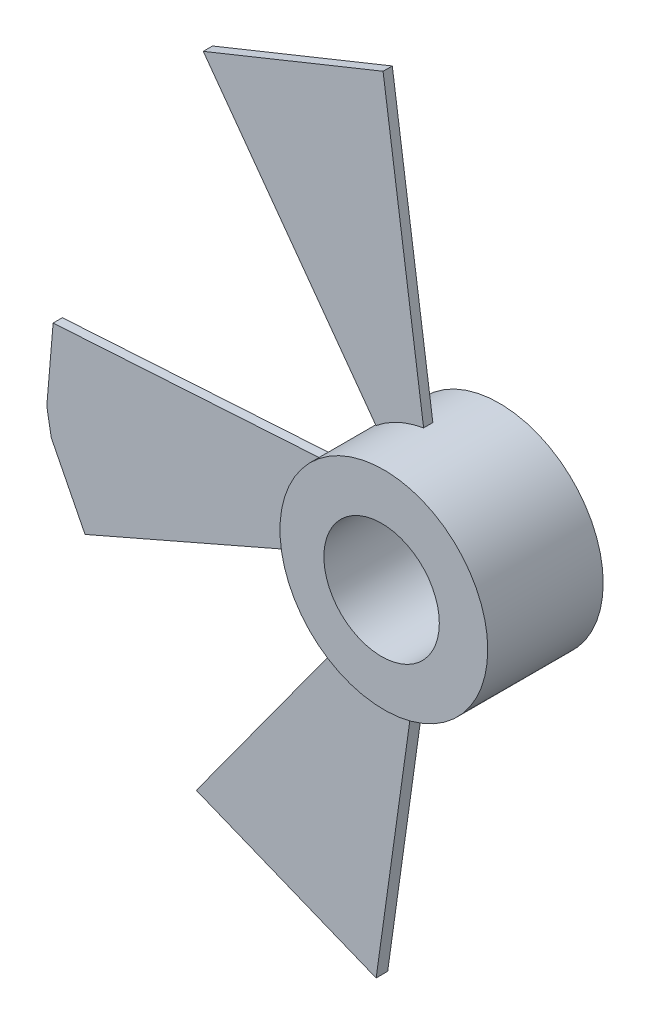
from build123d import *

# Parameters (mm, degrees)
EXTRUDE_1_DEPTH     = 4
EXTRUDE_1_2_DEPTH   = 4
EXTRUDE_1_3_DEPTH   = 4
SKETCH_2_R          = 90
SKETCH_2_R_2        = 57.5
EXTRUDE_2_DEPTH     = 50
SKETCH_4_R          = 57.5
SKETCH_4_R_2        = 50
EXTRUDE_3_DEPTH     = 100
CUT_EXTRUDE_1_DEPTH = 485.810454508
EXTRUDE_START       = 10
EXTRUDE_4_DEPTH     = 10


with BuildPart() as part:
    # 草图1 → 凸台-拉伸1 (new, symmetric)
    with BuildSketch(Plane.XY):
        with BuildLine():
            Line((-10.924807901, 55.668937127), (-50.690571005, 338.617043901))
            Line((-50.690571005, 338.617043901), (-206.438031879, 275.690985101))
            Line((-206.438031879, 275.690985101), (-37.918188894, 43.743319974))
            ThreePointArc((-37.918188894, 43.743319974), (-25.199590106, 51.467322598), (-10.924807901, 55.668937127))
        make_face()
    extrude(amount=EXTRUDE_1_DEPTH, both=True)



with BuildPart() as body_2:
    # 草图1 → Extrude 1 2 (new, symmetric)
    with BuildSketch(Plane.XY):
        with BuildLine():
            Line((-341.966631122, -58.160848878), (-338.146174396, -79.914727665))
            Line((-338.146174396, -79.914727665), (-308.839134252, -137.932805865))
            Line((-308.839134252, -137.932805865), (-53.490261468, -26.646674297))
            ThreePointArc((-53.490261468, -26.646674297), (-59.462925063, -1.128374922), (-53.490261468, 24.389924453))
            Line((-53.490261468, 24.389924453), (-336.508428621, 6.839151122))
            Line((-336.508428621, 6.839151122), (-341.966631122, -58.160848878))
        make_face()
    extrude(amount=EXTRUDE_1_2_DEPTH, both=True)


with BuildPart() as body_3:
    # 草图1 → Extrude 1 3 (new, symmetric)
    with BuildSketch(Plane.XY):
        with BuildLine():
            Line((-14.977351718, -57.136184189), (-46.962925063, -340))
            Line((-46.962925063, -340), (68.037074937, -340))
            Line((68.037074937, -340), (24.752563392, -52.045294277))
            ThreePointArc((24.752563392, -52.045294277), (5.345225431, -58.162057394), (-14.977351718, -57.136184189))
        make_face()
    extrude(amount=EXTRUDE_1_3_DEPTH, both=True)


with BuildPart() as part_1:
    add(part.part)

    add(body_2.part)  # 凸台-拉伸2 merges body 2

    add(body_3.part)  # 凸台-拉伸2 merges body 3
    # 草图2 → 凸台-拉伸2 (add, symmetric)
    with BuildSketch(Plane.XY.offset(4)):
        Circle(SKETCH_2_R)
        with Locations((-1.962925063, -1.128374922)):
            Circle(SKETCH_2_R_2, mode=Mode.SUBTRACT)
    extrude(amount=EXTRUDE_2_DEPTH, both=True)

    # 草图4 → 凸台-拉伸3 (add)
    with BuildSketch(Plane.XY.offset(54)):
        with Locations((-1.962925063, -1.128374922)):
            Circle(SKETCH_4_R)
        with Locations((-1.962925063, -1.128374922)):
            Circle(SKETCH_4_R_2, mode=Mode.SUBTRACT)
    extrude(amount=-EXTRUDE_3_DEPTH)

    # 草图7 → 切除-拉伸1 (cut, through all)
    with BuildSketch(Plane.XY.offset(4)):
        with BuildLine():
            Line((-18.476741558, -88.082972369), (-46.962925063, -340))
            Line((-46.962925063, -340), (68.037074937, -340))
            Line((68.037074937, -340), (29.699950595, -84.958301152))
            ThreePointArc((29.699950595, -84.958301152), (5.825032002, -89.811296629), (-18.476741558, -88.082972369))
        make_face()
    extrude(amount=-CUT_EXTRUDE_1_DEPTH, mode=Mode.SUBTRACT)

    # 草图9 → 凸台-拉伸4 (add)
    with BuildSketch(Plane.XY.offset(EXTRUDE_START)):
        with BuildLine():
            Line((-206.438031879, -275.690985101), (-56.836712635, -69.782434014))
            ThreePointArc((-56.836712635, -69.782434014), (-37.406446529, -81.858156332), (-15.559269973, -88.644848231))
            Line((-15.559269973, -88.644848231), (-50.690571005, -338.617043901))
            Line((-50.690571005, -338.617043901), (-206.438031879, -275.690985101))
        make_face()
    extrude(amount=-EXTRUDE_4_DEPTH)


solid = part_1.part
